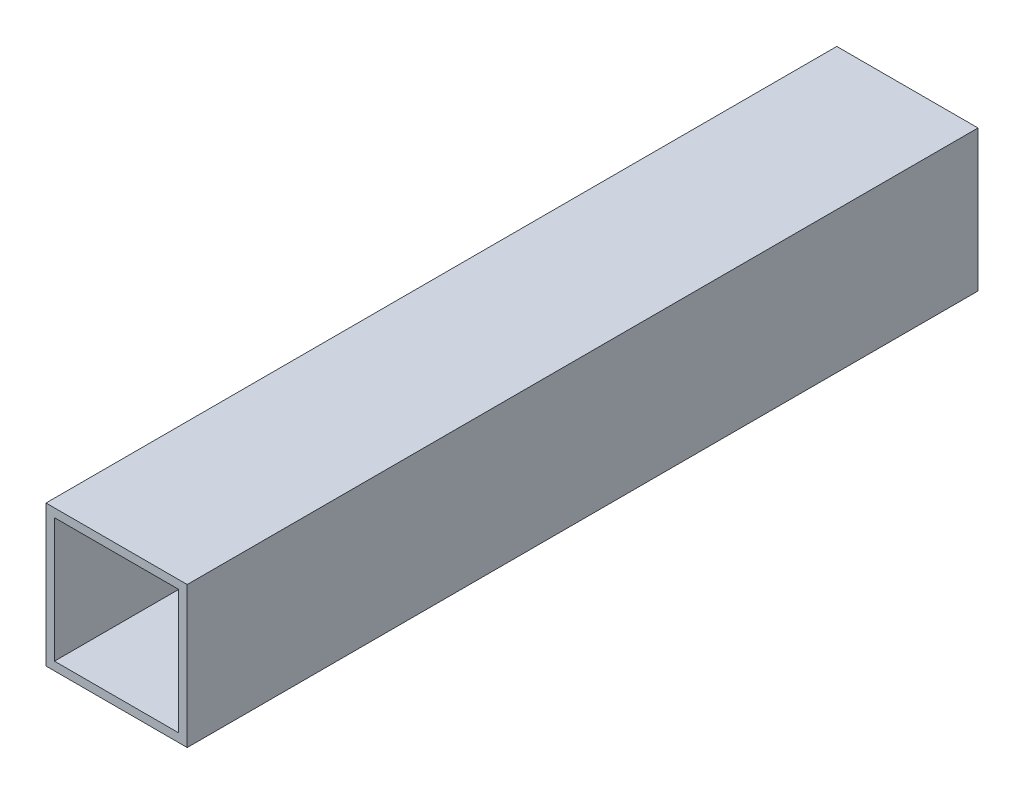
from build123d import *

# Parameters (mm, degrees)
SKETCH_1_W      = 50
SKETCH_1_H      = 50
SKETCH_1_W_2    = 44
SKETCH_1_H_2    = 44
EXTRUDE_2_DEPTH = 280


with BuildPart() as part:
    # 草图1 → 凸台-拉伸2 (new body)
    with BuildSketch(Plane.XY):
        with Locations((25, 25)):
            Rectangle(SKETCH_1_W, SKETCH_1_H)
        with Locations((25, 25)):
            Rectangle(SKETCH_1_W_2, SKETCH_1_H_2, mode=Mode.SUBTRACT)
    extrude(amount=EXTRUDE_2_DEPTH)


solid = part.part
